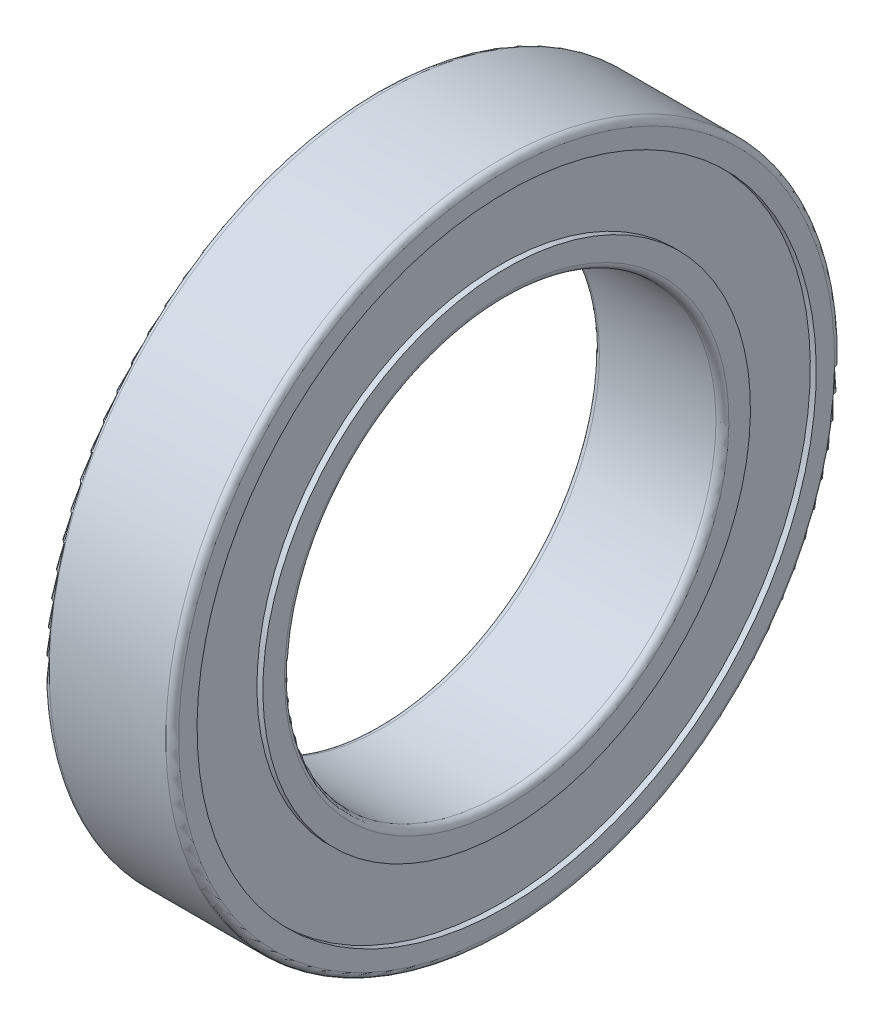
SolidWorks part; units mm, degrees
ref_plane "Front Plane" through (0, 0, 0) normal (0, 0, 1) x (1, 0, 0)
ref_plane "Top Plane" through (0, 0, 0) normal (0, 1, 0) x (1, 0, 0)
ref_plane "Right Plane" through (0, 0, 0) normal (1, 0, 0) x (0, 0, -1)
sketch "Sketch1" plane through (0, 0, 0) normal (0, 0, 1) x (1, 0, 0)
  line L0 (0, 0) -> (12, 0) construction
  line L1 (0, 20) -> (12, 20)
  line L2 (0, 31) -> (12, 31)
  line L3 (0, 31) -> (0, 28.7)
  line L4 (0, 28.7) -> (0.55, 28.7)
  line L5 (12, 31) -> (12, 28.7)
  line L6 (0.55, 28.7) -> (0.55, 22.6)
  line L7 (0.55, 22.6) -> (0, 22.6)
  line L8 (0, 22.6) -> (0, 20)
  line L9 (12, 28.7) -> (11.45, 28.7)
  line L10 (11.45, 28.7) -> (11.45, 22.6)
  line L11 (11.45, 22.6) -> (12, 22.6)
  line L12 (12, 22.6) -> (12, 20)
  dimension "D" = 62
  dimension "B" = 12
  dimension "D_s" = 40
  dimension "MSM_1" = 57.4
  dimension "MSM_2" = 45.2
  dimension "MSM_3" = 0.55
revolve "Revolve1" add sketch "Sketch1" angle 360 about L0
fillet "Fillet1" radius 0.6 2 edges at (12, -31, 0) (0, -31, 0)
fillet "Fillet2" radius 0.6 2 edges at (12, -20, 0) (0, -20, 0)
